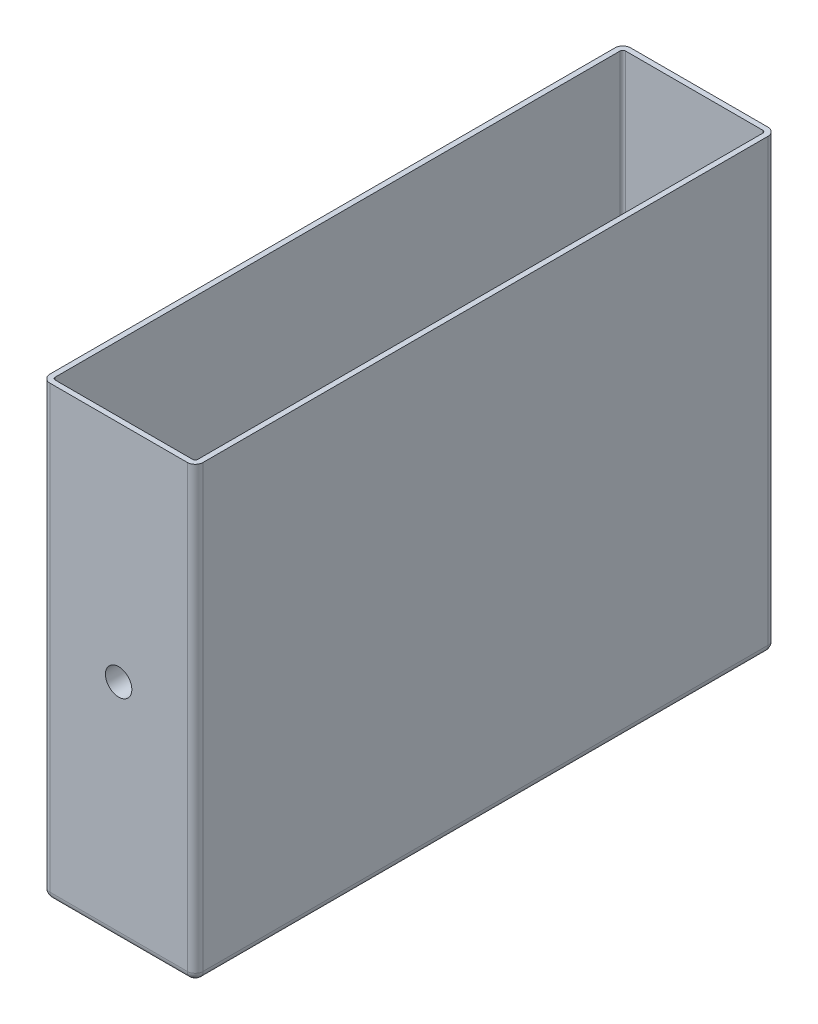
SolidWorks part; units mm, degrees
ref_plane "Front Plane" through (0, 0, 0) normal (0, 0, 1) x (1, 0, 0)
ref_plane "Top Plane" through (0, 0, 0) normal (0, 1, 0) x (1, 0, 0)
ref_plane "Right Plane" through (0, 0, 0) normal (1, 0, 0) x (0, 0, -1)
sketch "Sketch1" plane through (0, 0, 0) normal (0, 1, 0) x (1, 0, 0)
  line L1 (-14.5, 55) -> (14.5, 55)
  line L2 (-14.5, 55) -> (-14.5, -55)
  line L3 (-14.5, -55) -> (14.5, -55)
  line L4 (14.5, 55) -> (14.5, -55)
  line L5 (-14.5, 55) -> (14.5, -55) construction
  line L6 (-14.5, -55) -> (14.5, 55) construction
  point P0 (0, 0)
  dimension "D1" = 29
  dimension "D2" = 110
extrude "Boss-Extrude1" add sketch "Sketch1" along normal mid plane 85
fillet "Fillet1" radius 1.5 8 edges at (0, -42.5, -55) (14.5, -42.5, 0) (0, -42.5, 55) (-14.5, -42.5, 0) (-14.5, 0, -55) (14.5, 0, -55) (14.5, 0, 55) (-14.5, 0, 55)
shell "Shell1" thickness 1
sketch "Sketch2" plane through (0, 0, 54) normal (0, 0, -1) x (-1, 0, 0)
  circle A0 centre (0, 0) radius 5
  dimension "D1" = 10
extrude "Boss-Extrude2" add sketch "Sketch2" along normal blind 3
hole_wizard "M6 Tapped Hole1" positions "Sketch4" profile "Sketch3" tap size "M6" standard "Gb"
sketch "Sketch4" plane through (0, 0, 55) normal (0, 0, 1) x (1, 0, 0)
  point P0 (0, 0)
sketch "Sketch3" plane through (0, 0, 55) normal (1, 0, 0) x (0, -1, 0)
  line L0 (0, 0) -> (0, 4)
  line L1 (0, 4) -> (2.5, 4)
  line L2 (2.5, 4) -> (2.5, 0)
  line L5 (2.5, 0) -> (0, 0)
  line L11 (0, -6.35) -> (0, 107.95) construction
  dimension "通孔螺纹孔钻头直径" = 5
  dimension "通孔螺纹孔钻头深度" = 4
cosmetic thread "Cosmetic Thread1" parameters "D2"=6
